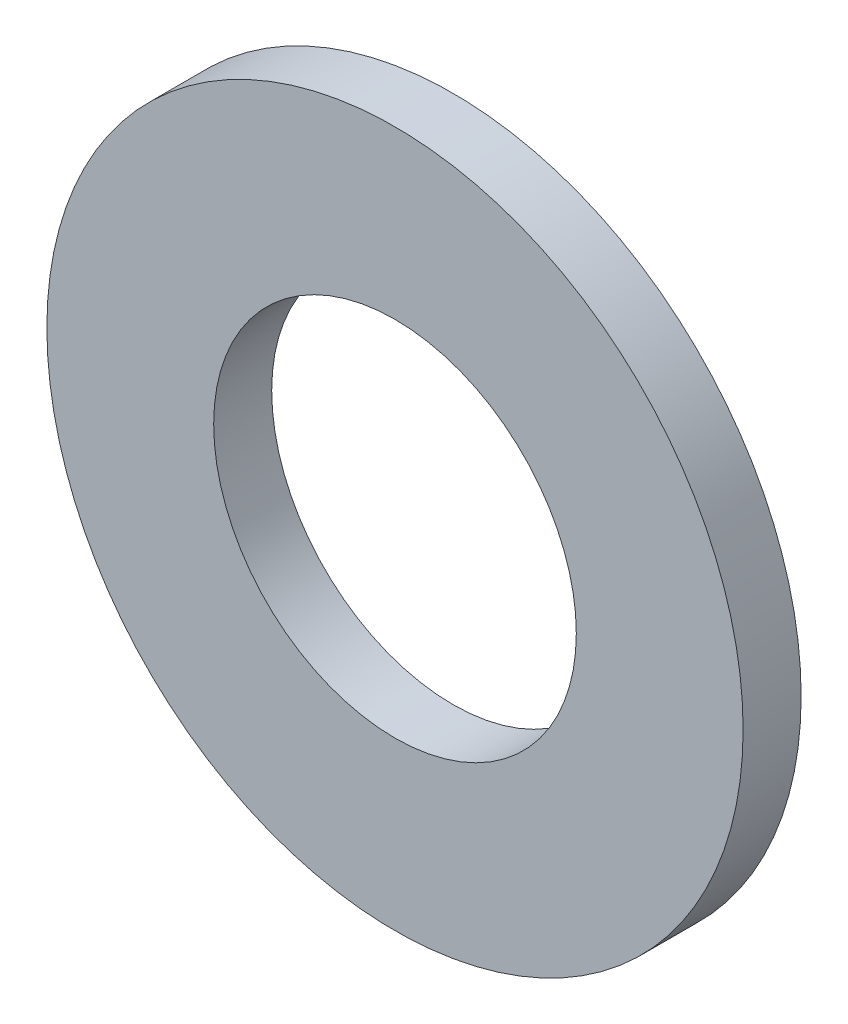
from build123d import *

# Parameters (mm, degrees)
SKETCH2_R           = 6
SKETCH2_R_2         = 3.125
BOSS_EXTRUDE1_DEPTH = 1


with BuildPart() as part:
    # Sketch2 → Boss-Extrude1 (new body)
    with BuildSketch(Plane.XY):
        Circle(SKETCH2_R)
        Circle(SKETCH2_R_2, mode=Mode.SUBTRACT)
    extrude(amount=BOSS_EXTRUDE1_DEPTH)


solid = part.part
